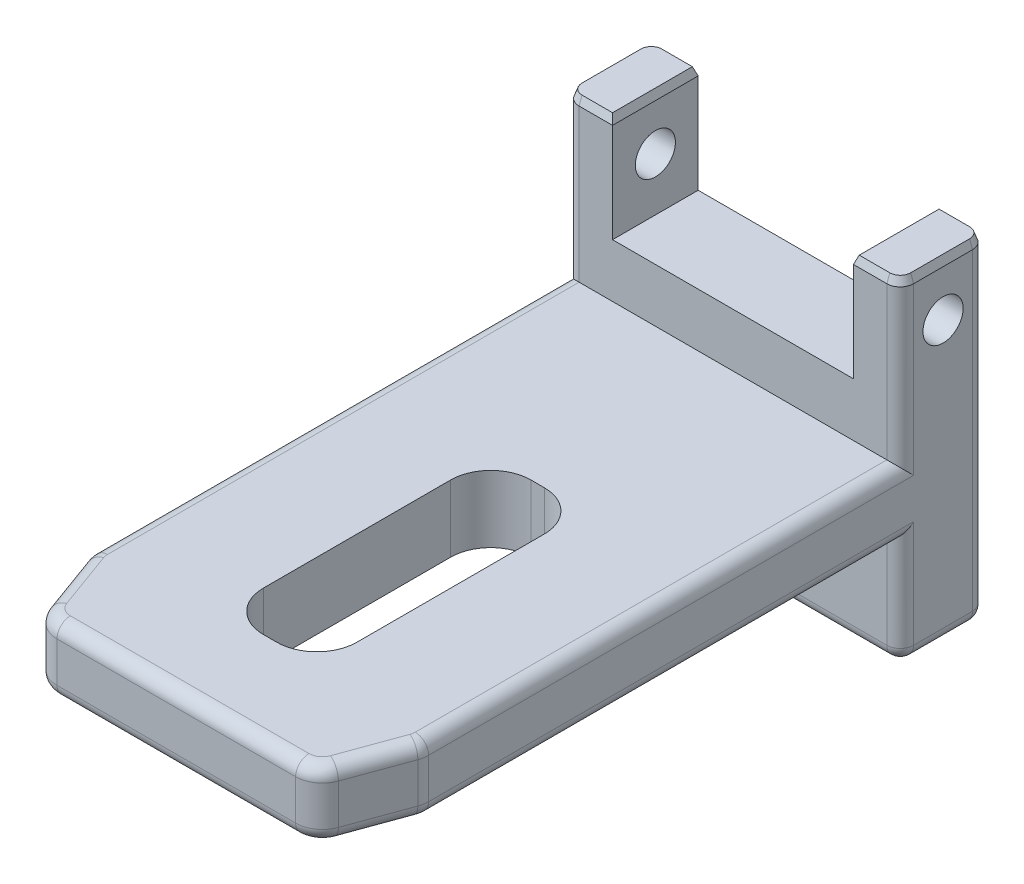
from build123d import *
from OCP.BRepFilletAPI import BRepFilletAPI_MakeChamfer

# Parameters (mm, degrees)
SKETCH1_W           = 12.5
SKETCH1_H           = 2.5
BOSS_EXTRUDE1_DEPTH = 24
SKETCH2_W           = 12.5
SKETCH2_H           = 3.2
BOSS_EXTRUDE2_DEPTH = 6
SKETCH3_R           = 0.75
CUT_EXTRUDE1_DEPTH  = 13
SKETCH4_W           = 9
SKETCH4_H           = 6.4
CUT_EXTRUDE2_DEPTH  = 4
SKETCH5_W           = 12.5
SKETCH5_H           = 3.2
BOSS_EXTRUDE3_DEPTH = 4
SKETCH7_W           = 3.5
SKETCH7_H           = 10
CUT_EXTRUDE3_DEPTH  = 4
FILLET3_R           = 1.5
CHAMFER1_SIZE       = 3
CHAMFER1_SIZE2      = 1.091910703
FILLET1_R           = 1
FILLET2_R           = 0.5
CHAMFER2_SIZE       = 0.3
CHAMFER2_SIZE2      = 0.10919107


with BuildPart() as part:
    # Sketch1 → Boss-Extrude1 (new body)
    with BuildSketch(Plane.XY):
        Rectangle(SKETCH1_W, SKETCH1_H)
    extrude(amount=BOSS_EXTRUDE1_DEPTH)

    # Sketch2 → Boss-Extrude2 (add)
    with BuildSketch(Plane(origin=(0, 1.25, 0), x_dir=(1, 0, 0), z_dir=(0, 1, 0))):
        with Locations((0, -1.6)):
            Rectangle(SKETCH2_W, SKETCH2_H)
    extrude(amount=BOSS_EXTRUDE2_DEPTH)

    # Sketch3 → Cut-Extrude1 (cut)
    with BuildSketch(Plane.ZY.offset(6.25)):
        with Locations((1.6, 5.23)):
            Circle(SKETCH3_R)
    extrude(amount=-CUT_EXTRUDE1_DEPTH, mode=Mode.SUBTRACT)

    # Sketch4 → Cut-Extrude2 (cut)
    with BuildSketch(Plane(origin=(0, 7.25, 0), x_dir=(1, 0, 0), z_dir=(0, 1, 0))):
        Rectangle(SKETCH4_W, SKETCH4_H)
    extrude(amount=-CUT_EXTRUDE2_DEPTH, mode=Mode.SUBTRACT)

    # Sketch5 → Boss-Extrude3 (add)
    with BuildSketch(Plane.XZ.offset(1.25)):
        with Locations((0, 1.6)):
            Rectangle(SKETCH5_W, SKETCH5_H)
    extrude(amount=BOSS_EXTRUDE3_DEPTH)

    # Sketch7 → Cut-Extrude3 (cut)
    with BuildSketch(Plane.XZ.offset(1.25)):
        with Locations((0, 15.5)):
            Rectangle(SKETCH7_W, SKETCH7_H)
    extrude(amount=-CUT_EXTRUDE3_DEPTH, mode=Mode.SUBTRACT)

    # Fillet3
    fillet3_edges = [part.edges().sort_by_distance(p)[0] for p in [
        (1.75, 0, 20.5),
        (1.75, 0, 10.5),
        (-1.75, 0, 10.5),
        (-1.75, 0, 20.5),
    ]]
    fillet(fillet3_edges, radius=FILLET3_R)

    # Chamfer1: one chamfer whose edges measure the first distance from different faces: ONE call of the kernel's chamfer builder (chamfer() names one face for all edges)
    chamfer1_edges_1 = [part.edges().sort_by_distance(p)[0] for p in [
        (-6.25, 0, 24),
    ]]
    chamfer1_side_1 = [part.faces().sort_by_distance(p)[0] for p in [
        (-6.25, 0.340871708, 8.515441233),
    ]]
    chamfer1_edges_2 = [part.edges().sort_by_distance(p)[0] for p in [
        (6.25, 0, 24),
    ]]
    chamfer1_side_2 = [part.faces().sort_by_distance(p)[0] for p in [
        (6.25, 0.340871708, 8.515441233),
    ]]
    chamfer1 = BRepFilletAPI_MakeChamfer(part.part.solid().wrapped)
    for e in chamfer1_edges_1:
        chamfer1.Add(CHAMFER1_SIZE, CHAMFER1_SIZE2, e.wrapped, chamfer1_side_1[0].wrapped)  # the first distance lies on this face
    for e in chamfer1_edges_2:
        chamfer1.Add(CHAMFER1_SIZE, CHAMFER1_SIZE2, e.wrapped, chamfer1_side_2[0].wrapped)  # the first distance lies on this face
    add(Compound.cast(chamfer1.Shape()), mode=Mode.REPLACE)

    # Fillet1
    fillet1_edges = [part.edges().sort_by_distance(p)[0] for p in [
        (-5.158089297, 0, 24),
        (5.158089297, 0, 24),
        (6.25, 0, 21),
        (-6.25, 0, 21),
    ]]
    fillet(fillet1_edges, radius=FILLET1_R)

    # Fillet2
    fillet2_edges = [part.edges().sort_by_distance(p)[0] for p in [
        (6.25, 1.25, 12.01183651),
        (6.25, -1.25, 12.01183651),
        (5.7936335, -1.25, 22.253856653),
        (0, -1.25, 24),
        (-5.7936335, -1.25, 22.253856653),
        (-6.25, -1.25, 12.01183651),
        (-5.031458195, -1.25, 23.819152044),
        (-6.234807753, -1.25, 20.997321197),
        (5.031458195, -1.25, 23.819152044),
        (6.234807753, -1.25, 20.997321197),
        (5.7936335, 1.25, 22.253856653),
        (0, 1.25, 24),
        (-6.25, 1.25, 12.01183651),
        (-5.7936335, 1.25, 22.253856653),
        (-5.031458195, 1.25, 23.819152044),
        (-6.234807753, 1.25, 20.997321197),
        (5.031458195, 1.25, 23.819152044),
        (6.234807753, 1.25, 20.997321197),
        (-6.25, 4.25, 3.2),
        (6.25, 4.25, 3.2),
        (-6.25, 1, 0),
        (-6.25, -3.25, 3.2),
        (6.25, -3.25, 3.2),
        (-6.25, -5.25, 1.6),
        (0, -5.25, 0),
        (6.25, -5.25, 1.6),
        (0, -5.25, 3.2),
        (6.25, 1, 0),
    ]]
    fillet(fillet2_edges, radius=FILLET2_R)

    # Chamfer2: one chamfer whose edges measure the first distance from different faces: ONE call of the kernel's chamfer builder (chamfer() names one face for all edges)
    chamfer2_edges_1 = [part.edges().sort_by_distance(p)[0] for p in [
        (-6.25, 7.25, 1.6),
    ]]
    chamfer2_side_1 = [part.faces().sort_by_distance(p)[0] for p in [
        (-6.25, 0.458482774, 6.931212407),
    ]]
    chamfer2_edges_2 = [part.edges().sort_by_distance(p)[0] for p in [
        (6.25, 7.25, 1.6),
    ]]
    chamfer2_side_2 = [part.faces().sort_by_distance(p)[0] for p in [
        (6.25, 0.458482774, 6.931212407),
    ]]
    chamfer2_edges_3 = [part.edges().sort_by_distance(p)[0] for p in [
        (5.125, 7.25, 0),
        (-5.125, 7.25, 0),
    ]]
    chamfer2_side_3 = [part.faces().sort_by_distance(p)[0] for p in [
        (0, -0.161764706, 0),
    ]]
    chamfer2_edges_4 = [part.edges().sort_by_distance(p)[0] for p in [
        (-5.125, 7.25, 3.2),
        (5.125, 7.25, 3.2),
    ]]
    chamfer2_side_4 = [part.faces().sort_by_distance(p)[0] for p in [
        (0, 3.159090909, 3.2),
    ]]
    chamfer2_edges_5 = [part.edges().sort_by_distance(p)[0] for p in [
        (6.103553391, 7.25, 0.146446609),
    ]]
    chamfer2_side_5 = [part.faces().sort_by_distance(p)[0] for p in [
        (6.103553391, 1.25, 0.146446609),
    ]]
    chamfer2_edges_6 = [part.edges().sort_by_distance(p)[0] for p in [
        (6.103553391, 7.25, 3.053553391),
    ]]
    chamfer2_side_6 = [part.faces().sort_by_distance(p)[0] for p in [
        (6.103553391, 4, 3.053553391),
    ]]
    chamfer2_edges_7 = [part.edges().sort_by_distance(p)[0] for p in [
        (-6.103553391, 7.25, 3.053553391),
    ]]
    chamfer2_side_7 = [part.faces().sort_by_distance(p)[0] for p in [
        (-6.103553391, 4, 3.053553391),
    ]]
    chamfer2_edges_8 = [part.edges().sort_by_distance(p)[0] for p in [
        (-6.103553391, 7.25, 0.146446609),
    ]]
    chamfer2_side_8 = [part.faces().sort_by_distance(p)[0] for p in [
        (-6.103553391, 1.25, 0.146446609),
    ]]
    chamfer2_edges_9 = [part.edges().sort_by_distance(p)[0] for p in [
        (4.5, 7.25, 1.6),
    ]]
    chamfer2_side_9 = [part.faces().sort_by_distance(p)[0] for p in [
        (4.5, 7.198775006, 1.6),
    ]]
    chamfer2_edges_10 = [part.edges().sort_by_distance(p)[0] for p in [
        (-4.5, 7.25, 1.6),
    ]]
    chamfer2_side_10 = [part.faces().sort_by_distance(p)[0] for p in [
        (-4.5, 7.198775006, 1.6),
    ]]
    chamfer2 = BRepFilletAPI_MakeChamfer(part.part.solid().wrapped)
    for e in chamfer2_edges_1:
        chamfer2.Add(CHAMFER2_SIZE, CHAMFER2_SIZE2, e.wrapped, chamfer2_side_1[0].wrapped)  # the first distance lies on this face
    for e in chamfer2_edges_2:
        chamfer2.Add(CHAMFER2_SIZE, CHAMFER2_SIZE2, e.wrapped, chamfer2_side_2[0].wrapped)  # the first distance lies on this face
    for e in chamfer2_edges_3:
        chamfer2.Add(CHAMFER2_SIZE, CHAMFER2_SIZE2, e.wrapped, chamfer2_side_3[0].wrapped)  # the first distance lies on this face
    for e in chamfer2_edges_4:
        chamfer2.Add(CHAMFER2_SIZE, CHAMFER2_SIZE2, e.wrapped, chamfer2_side_4[0].wrapped)  # the first distance lies on this face
    for e in chamfer2_edges_5:
        chamfer2.Add(CHAMFER2_SIZE, CHAMFER2_SIZE2, e.wrapped, chamfer2_side_5[0].wrapped)  # the first distance lies on this face
    for e in chamfer2_edges_6:
        chamfer2.Add(CHAMFER2_SIZE, CHAMFER2_SIZE2, e.wrapped, chamfer2_side_6[0].wrapped)  # the first distance lies on this face
    for e in chamfer2_edges_7:
        chamfer2.Add(CHAMFER2_SIZE, CHAMFER2_SIZE2, e.wrapped, chamfer2_side_7[0].wrapped)  # the first distance lies on this face
    for e in chamfer2_edges_8:
        chamfer2.Add(CHAMFER2_SIZE, CHAMFER2_SIZE2, e.wrapped, chamfer2_side_8[0].wrapped)  # the first distance lies on this face
    for e in chamfer2_edges_9:
        chamfer2.Add(CHAMFER2_SIZE, CHAMFER2_SIZE2, e.wrapped, chamfer2_side_9[0].wrapped)  # the first distance lies on this face
    for e in chamfer2_edges_10:
        chamfer2.Add(CHAMFER2_SIZE, CHAMFER2_SIZE2, e.wrapped, chamfer2_side_10[0].wrapped)  # the first distance lies on this face
    add(Compound.cast(chamfer2.Shape()), mode=Mode.REPLACE)


solid = part.part
